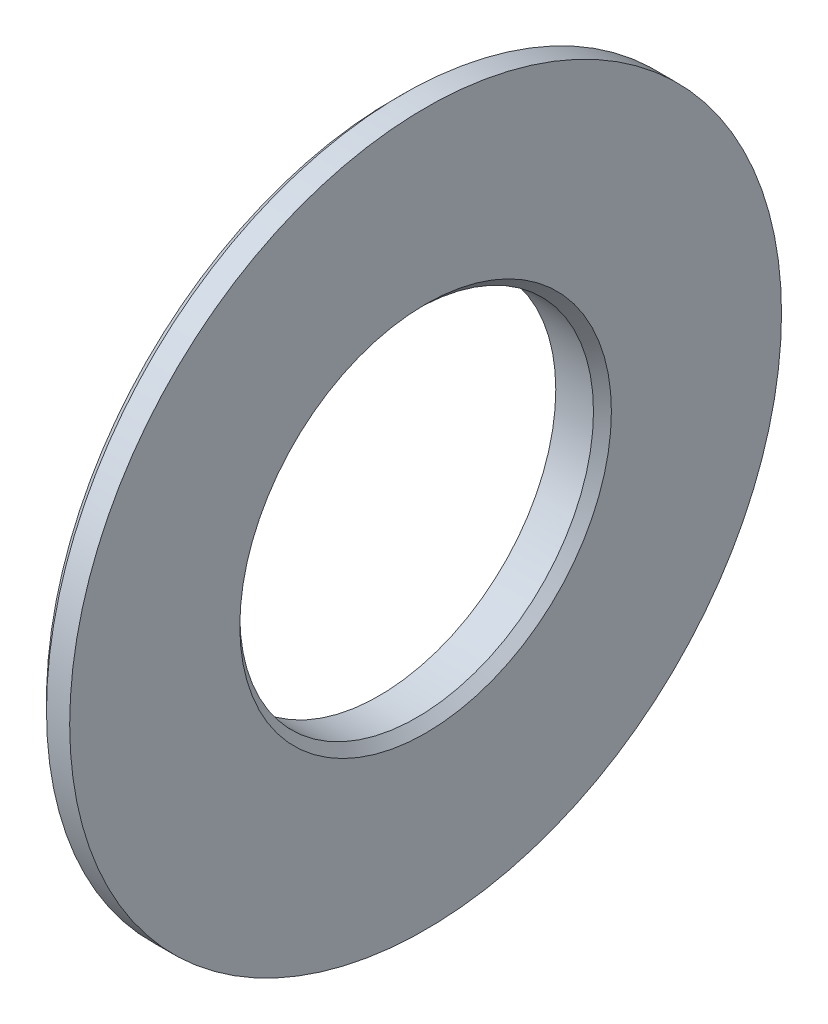
from build123d import *

# Parameters (mm, degrees)
CHAMFER_1_SIZE = 1
CHAMFER_2_SIZE = 1


with BuildPart() as part:
    # 草图1 → 旋转1 (revolve)
    with BuildSketch(Plane.XY, mode=Mode.PRIVATE) as revolve_1_sk:
        Polygon((6.503433875, -2.666983759), (6.503433875, 2.333016241), (8.12324826, 2.333016241), (8.12324826, 17.333016241), (11.713433875, 17.333016241), (11.713433875, -2.666983759), align=None)
    revolve(revolve_1_sk.sketch.rotate(Axis((4.025427808, -22.416983759, 0), (1, 0, 0)), 90), axis=Axis((4.025427808, -22.416983759, 0), (1, 0, 0)))

    # 倒角1
    chamfer_1_edges = [part.edges().sort_by_distance(p)[0] for p in [
        (8.12324826, -22.416983759, -39.75),
    ]]
    chamfer(chamfer_1_edges, length=CHAMFER_1_SIZE)

    # 倒角2
    chamfer_2_edges = [part.edges().sort_by_distance(p)[0] for p in [
        (11.713433875, -22.416983759, -19.75),
    ]]
    chamfer(chamfer_2_edges, length=CHAMFER_2_SIZE)


solid = part.part
